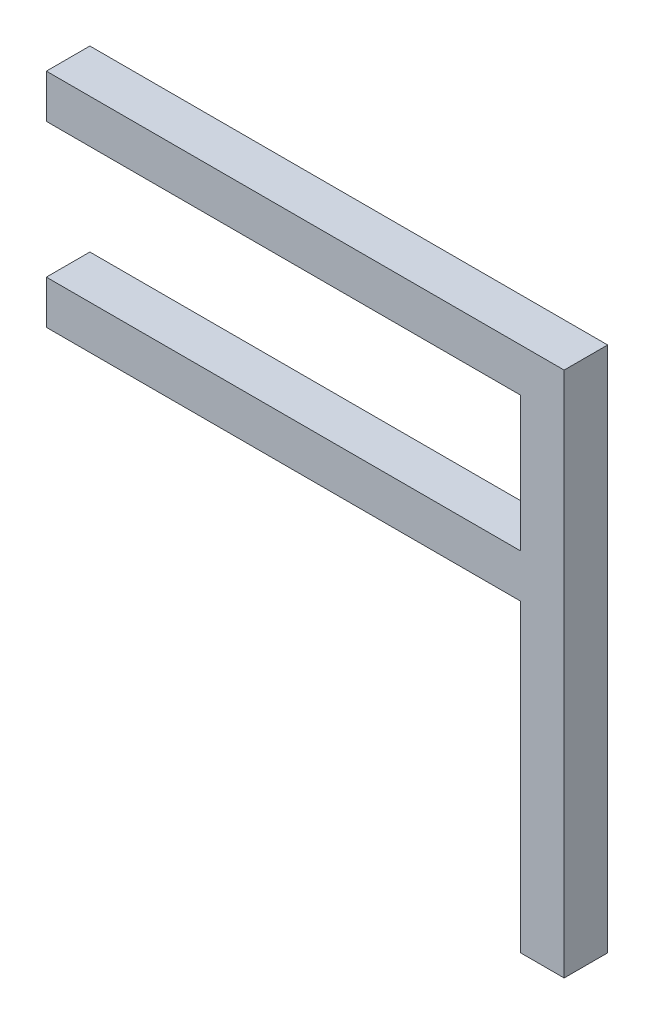
SolidWorks part; units mm, degrees
ref_plane "前视基准面" through (0, 0, 0) normal (0, 0, 1) x (1, 0, 0)
ref_plane "上视基准面" through (0, 0, 0) normal (0, 1, 0) x (1, 0, 0)
ref_plane "右视基准面" through (0, 0, 0) normal (1, 0, 0) x (0, 0, -1)
sketch "草图1" plane through (0, 0, 0) normal (0, 0, 1) x (1, 0, 0)
  line L0 (0, 0) -> (570, 0)
  line L1 (570, 0) -> (570, 545)
  line L2 (570, 545) -> (0, 545)
  line L3 (0, 545) -> (0, 0)
  line L4 (50, 50) -> (520, 50)
  line L5 (520, 50) -> (520, 495)
  line L6 (520, 495) -> (50, 495)
  line L7 (50, 495) -> (50, 50)
  dimension "D1" = 50
extrude "凸台-拉伸1" add sketch "草图1" along normal blind 50
sketch "草图2" plane through (0, 0, 0) normal (0, 0, -1) x (-1, 0, 0)
  line L2 (-520, 290) -> (-50, 290)
  line L3 (-50, 495) -> (-50, 50) construction
  line L4 (-50, 290) -> (-50, 340)
  line L5 (-50, 340) -> (-520, 340)
  line L6 (-520, 50) -> (-520, 495) construction
  line L7 (-520, 340) -> (-520, 290)
extrude "凸台-拉伸2" add sketch "草图2" against normal blind 50
sketch "草图3" plane through (0, 0, 0) normal (0, -1, 0) x (1, 0, 0)
  line L0 (0, 50) -> (0, 0)
  line L1 (0, 0) -> (50, 0)
  line L2 (50, 0) -> (50, 50)
  line L3 (0, 50) -> (570, 50) construction
  line L4 (50, 50) -> (0, 50)
  line L5 (570, 50) -> (520, 50)
  line L6 (520, 50) -> (520, 0)
  line L7 (0, 0) -> (570, 0) construction
  line L8 (520, 0) -> (570, 0)
  line L9 (570, 0) -> (570, 50)
extrude "凸台-拉伸3" add sketch "草图3" along normal blind 50
sketch "草图4" plane through (0, 0, 50) normal (0, 0, 1) x (1, 0, 0)
  line L0 (50, 50) -> (50, 0)
  line L1 (50, 0) -> (520, 0)
  line L2 (520, 0) -> (520, 50)
  line L3 (520, 50) -> (50, 50)
extrude "切除-拉伸1" cut sketch "草图4" against normal blind 50
sketch "草图5" plane through (520, 0, 0) normal (-1, 0, 0) x (0, 0, 1)
  line L0 (50, -50) -> (0, -50)
  line L1 (0, -50) -> (0, 0)
  line L2 (0, 0) -> (50, 0)
  line L3 (50, -50) -> (50, 290) construction
  line L4 (50, 0) -> (50, -10.3257)
  line L5 (50, -50) -> (50, -10.3257)
extrude "凸台-拉伸4" add sketch "草图5" along normal blind 478
sketch "草图6" plane through (0, 0, 50) normal (0, 0, 1) x (1, 0, 0)
  line L0 (0, -50) -> (0, 0)
  line L1 (0, 0) -> (570, 0)
  line L2 (570, -50) -> (570, 545) construction
  line L3 (570, 0) -> (570, -50)
  line L4 (570, -50) -> (0, -50)
extrude "切除-拉伸2" cut sketch "草图6" against normal blind 76
sketch "草图7" plane through (0, 0, 0) normal (-1, 0, 0) x (0, 0, 1)
  line L8 (0, 545) -> (0, 0)
  line L9 (0, 0) -> (50, 0)
  line L10 (50, 0) -> (50, 545)
  line L11 (50, 545) -> (0, 545)
  line L12 (0, 545) -> (0, 0)
  line L13 (0, 0) -> (50, 0)
  line L14 (50, 0) -> (50, 545)
  line L15 (50, 545) -> (0, 545)
  dimension "D1" = 0
extrude "凸台-拉伸5" add sketch "草图7" against normal blind 50
sketch "草图8" plane through (0, 0, 0) normal (-1, 0, 0) x (0, 0, 1)
  line L8 (0, 545) -> (0, 0)
  line L9 (0, 0) -> (50, 0)
  line L10 (50, 0) -> (50, 545)
  line L11 (50, 545) -> (0, 545)
  line L12 (0, 545) -> (0, 0)
  line L13 (0, 0) -> (50, 0)
  line L14 (50, 0) -> (50, 545)
  line L15 (50, 545) -> (0, 545)
  dimension "D1" = 0
extrude "切除-拉伸3" cut sketch "草图8" against normal blind 50
sketch "草图9" plane through (50, 0, 0) normal (-1, 0, 0) x (0, 0, 1)
  line L8 (50, 495) -> (50, 545)
  line L9 (50, 545) -> (0, 545)
  line L10 (0, 545) -> (0, 495)
  line L11 (0, 495) -> (50, 495)
  line L12 (50, 495) -> (50, 545)
  line L13 (50, 545) -> (0, 545)
  line L14 (0, 545) -> (0, 495)
  line L15 (0, 495) -> (50, 495)
  line L20 (50, 290) -> (50, 340)
  line L21 (50, 340) -> (0, 340)
  line L22 (0, 340) -> (0, 290)
  line L23 (0, 290) -> (50, 290)
  line L24 (50, 290) -> (50, 340)
  line L25 (50, 340) -> (0, 340)
  line L26 (0, 340) -> (0, 290)
  line L27 (0, 290) -> (50, 290)
  dimension "D1" = 0
  dimension "D2" = 0
extrude "凸台-拉伸6" add sketch "草图9" along normal blind 20
sketch "草图10" plane through (30, 0, 0) normal (-1, 0, 0) x (0, 0, 1)
  line L8 (0, 495) -> (50, 495)
  line L9 (50, 495) -> (50, 545)
  line L10 (50, 545) -> (0, 545)
  line L11 (0, 545) -> (0, 495)
  line L12 (0, 495) -> (50, 495)
  line L13 (50, 495) -> (50, 545)
  line L14 (50, 545) -> (0, 545)
  line L15 (0, 545) -> (0, 495)
  line L20 (0, 290) -> (50, 290)
  line L21 (50, 290) -> (50, 340)
  line L22 (50, 340) -> (0, 340)
  line L23 (0, 340) -> (0, 290)
  line L24 (0, 290) -> (50, 290)
  line L25 (50, 290) -> (50, 340)
  line L26 (50, 340) -> (0, 340)
  line L27 (0, 340) -> (0, 290)
  dimension "D1" = 0
  dimension "D2" = 0
extrude "凸台-拉伸7" add sketch "草图10" along normal blind 10
sketch "草图11" plane through (0, 0, 0) normal (0, -1, 0) x (1, 0, 0)
  line L8 (520, 50) -> (520, 0)
  line L9 (520, 0) -> (570, 0)
  line L10 (570, 0) -> (570, 50)
  line L11 (570, 50) -> (520, 50)
  line L12 (520, 50) -> (520, 0)
  line L13 (520, 0) -> (570, 0)
  line L14 (570, 0) -> (570, 50)
  line L15 (570, 50) -> (520, 50)
  dimension "D1" = 0
extrude "凸台-拉伸8" add sketch "草图11" along normal blind 60
sketch "草图12" plane through (20, 0, 0) normal (-1, 0, 0) x (0, 0, 1)
  line L8 (0, 545) -> (0, 495)
  line L9 (0, 495) -> (50, 495)
  line L10 (50, 495) -> (50, 545)
  line L11 (50, 545) -> (0, 545)
  line L12 (0, 545) -> (0, 495)
  line L13 (0, 495) -> (50, 495)
  line L14 (50, 495) -> (50, 545)
  line L15 (50, 545) -> (0, 545)
  line L20 (0, 340) -> (0, 290)
  line L21 (0, 290) -> (50, 290)
  line L22 (50, 290) -> (50, 340)
  line L23 (50, 340) -> (0, 340)
  line L24 (0, 340) -> (0, 290)
  line L25 (0, 290) -> (50, 290)
  line L26 (50, 290) -> (50, 340)
  line L27 (50, 340) -> (0, 340)
  dimension "D1" = 0
  dimension "D2" = 0
extrude "凸台-拉伸9" add sketch "草图12" along normal blind 45
